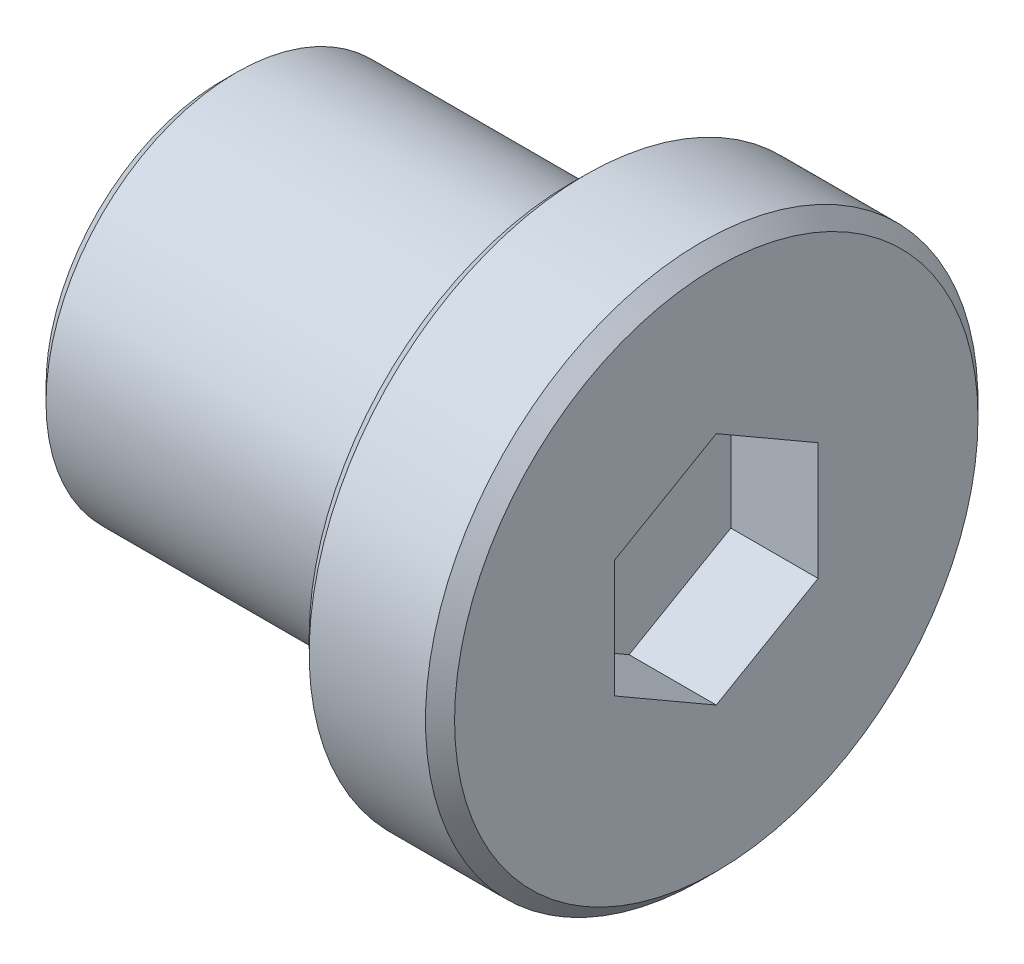
SolidWorks part; units mm, degrees
ref_plane "Front Plane" through (0, 0, 0) normal (0, 0, 1) x (1, 0, 0)
ref_plane "Top Plane" through (0, 0, 0) normal (0, 1, 0) x (1, 0, 0)
ref_plane "Right Plane" through (0, 0, 0) normal (1, 0, 0) x (0, 0, -1)
sketch "Sketch1" plane through (0, 0, 0) normal (0, 0, 1) x (1, 0, 0)
  line L0 (0, 0) -> (0, 6.55)
  line L1 (0, 6.55) -> (12, 6.55)
  line L2 (12, 6.55) -> (12, 9.5)
  line L3 (12, 9.5) -> (17, 9.5)
  line L4 (17, 9.5) -> (17, 0)
  line L5 (17, 0) -> (0, 0)
  dimension "D1" = 6.55
  dimension "D2" = 12
  dimension "D3" = 17
  dimension "D4" = 9.5
revolve "Revolve1" add sketch "Sketch1" angle 360 about L5
cosmetic thread "Cosmetic Thread1" parameters "D2"=11.445
sketch "Sketch2" plane through (17, 0, 0) normal (1, 0, 0) x (0, 0, -1)
  line L1 (0, 4.0415) -> (-3.5, 2.0207)
  line L2 (-3.5, 2.0207) -> (-3.5, -2.0207)
  line L3 (-3.5, -2.0207) -> (0, -4.0415)
  line L4 (0, -4.0415) -> (3.5, -2.0207)
  line L5 (3.5, -2.0207) -> (3.5, 2.0207)
  line L6 (3.5, 2.0207) -> (0, 4.0415)
  circle A0 centre (0, 0) radius 3.5 construction
  dimension "D1" = 7
extrude "Cut-Extrude1" cut sketch "Sketch2" against normal blind 3
chamfer "Chamfer1" distance 0.5 angle 45 3 edges at (17, 9.5, 0) (12, 9.5, 0) (0, 6.55, 0)
